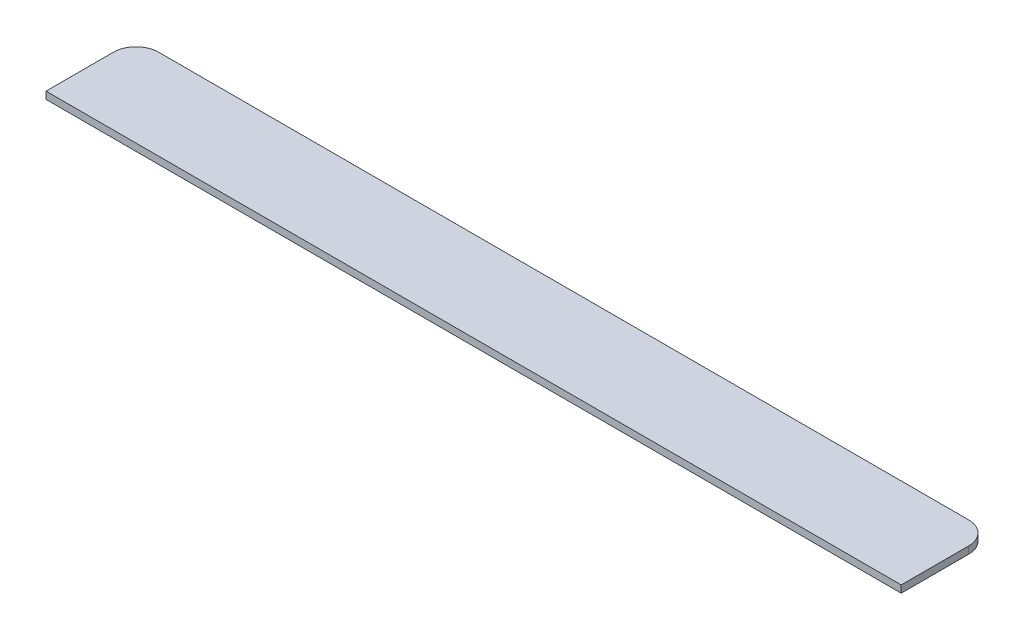
from build123d import *

# Parameters (mm, degrees)
BOSS_EXTRUDE1_DEPTH = 1.6


with BuildPart() as part:
    # Sketch1 → Boss-Extrude1 (new body)
    with BuildSketch(Plane(origin=(0, 0, 0), x_dir=(1, 0, 0), z_dir=(0, 1, 0))):
        with BuildLine():
            Line((0, 0), (190, 0))
            Line((190, 0), (190, 15))
            ThreePointArc((190, 15), (188.535533906, 18.535533906), (185, 20))
            Line((185, 20), (5, 20))
            ThreePointArc((5, 20), (1.464466094, 18.535533906), (0, 15))
            Line((0, 15), (0, 0))
        make_face()
    extrude(amount=BOSS_EXTRUDE1_DEPTH)


solid = part.part
